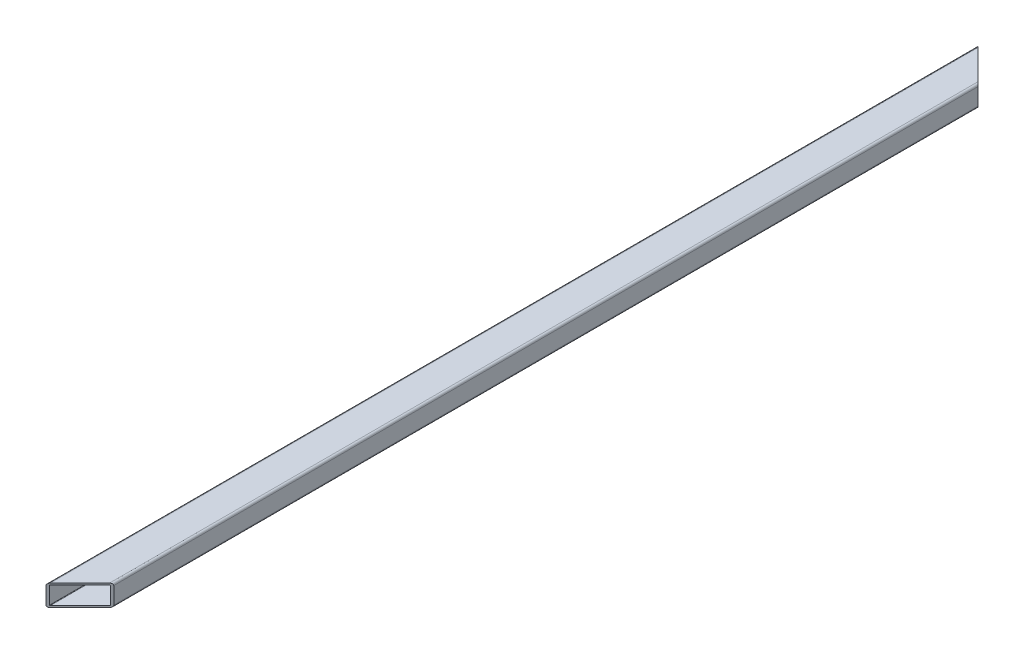
SolidWorks part; units mm, degrees
material "1023 Carbon Steel Plate (SS)"
ref_plane "Front Plane" through (0, 0, 0) normal (0, 0, 1) x (1, 0, 0)
ref_plane "Top Plane" through (0, 0, 0) normal (0, 1, 0) x (1, 0, 0)
ref_plane "Right Plane" through (0, 0, 0) normal (1, 0, 0) x (0, 0, -1)
sketch "Sketch1" plane through (0, 0, 0) normal (0, 0, 1) x (1, 0, 0)
  line L1 (35, 25) -> (-35, 25)
  line L2 (40, 20) -> (40, -20)
  line L3 (35, -25) -> (-35, -25)
  line L4 (-40, 20) -> (-40, -20)
  line L5 (40, 25) -> (-40, -25) construction
  line L6 (40, -25) -> (-40, 25) construction
  arc A0 (-35, -25) -> (-40, -20) centre (-35, -20) cw
  arc A1 (40, -20) -> (35, -25) centre (35, -20) cw
  arc A2 (35, 25) -> (40, 20) centre (35, 20) cw
  arc A3 (-35, 25) -> (-40, 20) centre (-35, 20) ccw
  point P0 (0, 0)
  dimension "D3" = 5
  dimension "D1" = 80
  dimension "D2" = 50
extrude "Boss-Extrude1" add sketch "Sketch1" along normal blind 2200 contours L4 A0 L3 A1 L2 A2 L1 A3
shell "Shell1" thickness 4
sketch "Sketch3" plane through (0, -25, 0) normal (0, -1, 0) x (1, 0, 0)
  line L0 (-40, 2200) -> (40, 2120)
  line L1 (40, 2200) -> (40, 0) construction
  line L2 (40, 2120) -> (40, 2200)
  line L3 (40, 2200) -> (-40, 2200)
  line L4 (-35, 1100) -> (784.0884, 1100) construction
  line L5 (-35, 2200) -> (-35, 0) construction
  line L6 (-40, 2200) -> (-40, 0) construction
  line L7 (40, 80) -> (40, 0)
  line L8 (-40, 0) -> (40, 80)
  line L9 (40, 0) -> (-40, 0)
  dimension "D1" = 45
extrude "Cut-Extrude2" cut sketch "Sketch3" against normal blind 2000
